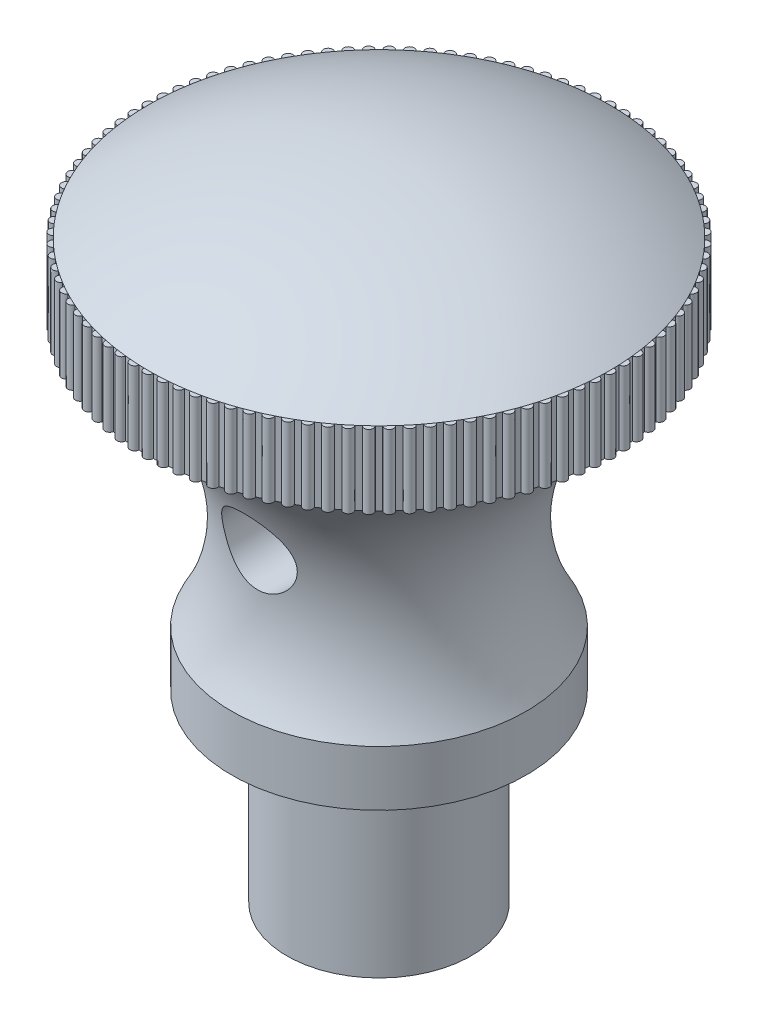
from build123d import *

# Parameters (mm, degrees)
SKETCH8_R           = 2
CUT_EXTRUDE4_DEPTH  = 10
SKETCH9_R           = 0.25
BOSS_EXTRUDE2_DEPTH = 4
CIRPATTERN3_COUNT   = 100
SKETCH10_R          = 2
CUT_EXTRUDE6_DEPTH  = 22


with BuildPart() as part:
    # Sketch7 → Revolve3 (revolve)
    with BuildSketch(Plane.XY, mode=Mode.PRIVATE) as revolve3_sk:
        with BuildLine():
            Line((0, 35), (0, 0))
            Line((0, 0), (5, 0))
            Line((5, 0), (5, 10))
            Line((5, 10), (8, 10))
            Line((8, 10), (8, 13))
            ThreePointArc((8, 13), (7.049202885, 21.137928329), (12.5, 27.255011249))
            Line((12.5, 27.255011249), (12.5, 31.255011249))
            ThreePointArc((12.5, 31.255011249), (6.524472024, 34.043636626), (0, 35))
        make_face()
    revolve(revolve3_sk.sketch.rotate(Axis((0, 0, 0), (0, 1, 0)), 90), axis=Axis((0, 0, 0), (0, 1, 0)))

    # Sketch8 → Cut-Extrude4 (cut, symmetric)
    with BuildSketch(Plane.XY):
        with Locations(Location((0, 20, 0), (0, 0, 270.000000125))):
            Circle(SKETCH8_R)
    extrude(amount=CUT_EXTRUDE4_DEPTH, both=True, mode=Mode.SUBTRACT)

    # Sketch9 → Boss-Extrude2 (add)
    with BuildSketch(Plane(origin=(0, 27.255011249, 0), x_dir=(-1, 0, 0), z_dir=(0, -1, 0))):
        with Locations((-12.5, 0)):
            Circle(SKETCH9_R)
    boss_extrude2 = extrude(amount=-BOSS_EXTRUDE2_DEPTH)

    # CirPattern3: Boss-Extrude2 ×100 about axis
    cirpattern3_axis = Axis((0, 0, 0), (0, 1, 0))
    for i in range(1, CIRPATTERN3_COUNT):
        add(boss_extrude2.rotate(cirpattern3_axis, i * 360 / CIRPATTERN3_COUNT))

    # Sketch10 → Cut-Extrude6 (cut)
    with BuildSketch(Plane.XZ):
        with Locations(Location((0, 0, 0), (0, 0, 270))):
            Circle(SKETCH10_R)
    extrude(amount=-CUT_EXTRUDE6_DEPTH, mode=Mode.SUBTRACT)


solid = part.part
